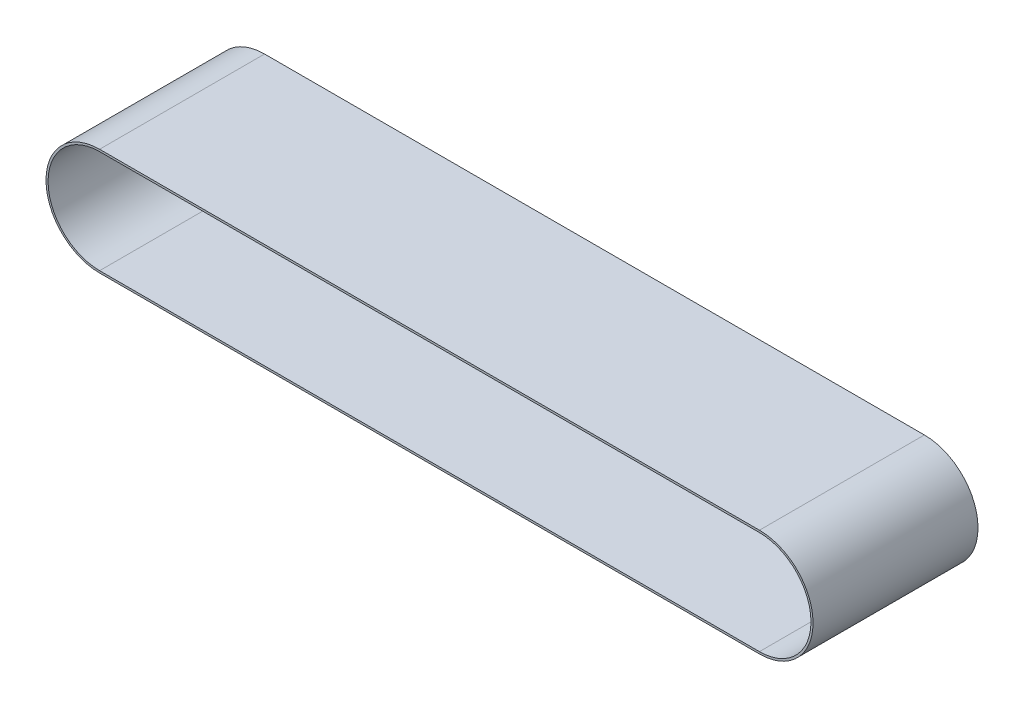
SolidWorks part; units mm, degrees
ref_plane "Front Plane" through (0, 0, 0) normal (0, 0, 1) x (1, 0, 0)
ref_plane "Top Plane" through (0, 0, 0) normal (0, 1, 0) x (1, 0, 0)
ref_plane "Right Plane" through (0, 0, 0) normal (1, 0, 0) x (0, 0, -1)
sketch "Sketch1" plane through (0, 0, 0) normal (0, 0, 1) x (1, 0, 0)
  line L0 (0, 0) -> (320, 0) construction
  line L1 (0, 25) -> (320, 25)
  line L2 (320, -25) -> (0, -25)
  line L3 (320, -26) -> (0, -26)
  line L4 (0, 26) -> (320, 26)
  arc A0 (0, 25) -> (0, -25) centre (0, 0) ccw
  arc A1 (320, -25) -> (320, 25) centre (320, 0) ccw
  arc A2 (0, 26) -> (0, -26) centre (0, 0) ccw
  arc A3 (320, -26) -> (320, 26) centre (320, 0) ccw
  dimension "D2" = 50
  dimension "D3" = 50
  dimension "D1" = 320
  dimension "D4" = 1
extrude "Boss-Extrude1" add sketch "Sketch1" along normal blind 80
